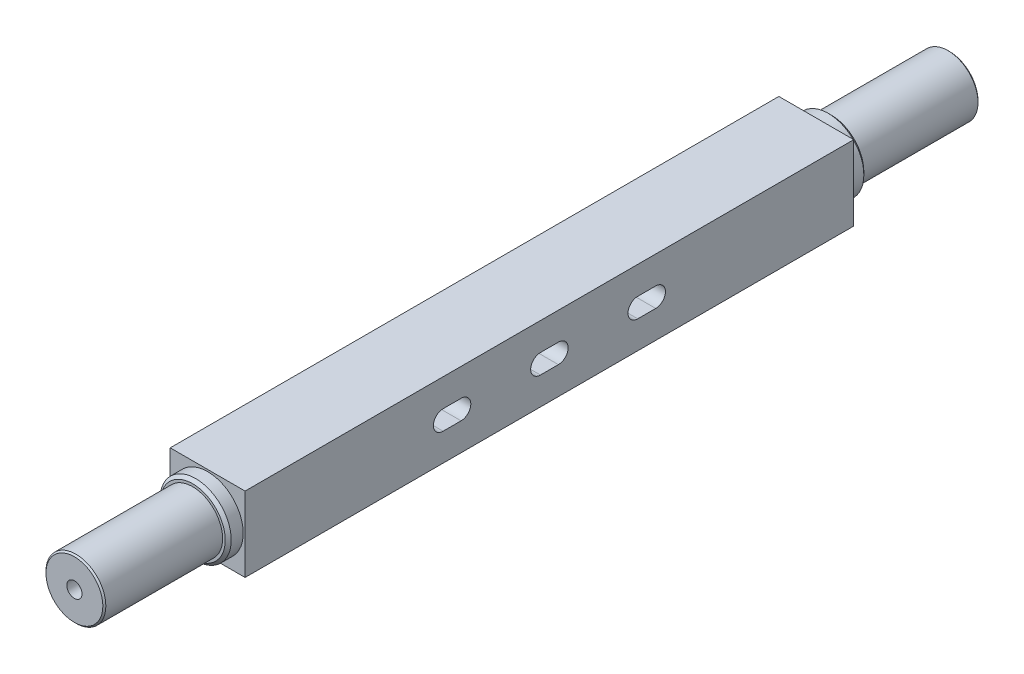
from build123d import *

# Parameters (mm, degrees)
SKETCH_1_R              = 20
EXTRUDE_1_DEPTH         = 79
SKETCH_2_R              = 23.75
EXTRUDE_2_DEPTH         = 10
CHAMFER_1_SIZE          = 2
SKETCH_3_W              = 50
SKETCH_3_H              = 50
EXTRUDE_3_DEPTH         = 406.5
SKETCH_4_R              = 23.75
EXTRUDE_4_DEPTH         = 10
CHAMFER_2_SIZE          = 2
SKETCH_5_R              = 20
EXTRUDE_5_DEPTH         = 79
CHAMFER_3_SIZE          = 1
HOLE_WIZARD_M12_1_D     = 10.2
HOLE_WIZARD_M12_1_DEPTH = 29.25
HOLE_WIZARD_M12_1_TIP   = 3.064389157
HOLE_WIZARD_M12_2_D     = 10.2
HOLE_WIZARD_M12_2_DEPTH = 29.25
HOLE_WIZARD_M12_2_TIP   = 3.064389157
CUT_EXTRUDE_1_DEPTH     = 79


with BuildPart() as part:
    # 草图1 → 凸台-拉伸1 (new body)
    with BuildSketch(Plane.XY):
        Circle(SKETCH_1_R)
    extrude(amount=EXTRUDE_1_DEPTH)

    # 草图2 → 凸台-拉伸2 (add)
    with BuildSketch(Plane.XY.offset(79)):
        Circle(SKETCH_2_R)
    extrude(amount=EXTRUDE_2_DEPTH)

    # 倒角1
    chamfer_1_edges = [part.edges().sort_by_distance(p)[0] for p in [
        (-23.75, 0, 79),
    ]]
    chamfer(chamfer_1_edges, length=CHAMFER_1_SIZE)

    # 草图3 → 凸台-拉伸3 (add)
    with BuildSketch(Plane.XY.offset(89)):
        Rectangle(SKETCH_3_W, SKETCH_3_H)
    extrude(amount=EXTRUDE_3_DEPTH)

    # 草图4 → 凸台-拉伸4 (add)
    with BuildSketch(Plane.XY.offset(495.5)):
        Circle(SKETCH_4_R)
    extrude(amount=EXTRUDE_4_DEPTH)

    # 倒角2
    chamfer_2_edges = [part.edges().sort_by_distance(p)[0] for p in [
        (-23.75, 0, 505.5),
    ]]
    chamfer(chamfer_2_edges, length=CHAMFER_2_SIZE)

    # 草图5 → 凸台-拉伸5 (add)
    with BuildSketch(Plane.XY.offset(505.5)):
        Circle(SKETCH_5_R)
    extrude(amount=EXTRUDE_5_DEPTH)

    # 倒角3
    chamfer_3_edges = [part.edges().sort_by_distance(p)[0] for p in [
        (-20, 0, 0),
        (-20, 0, 584.5),
    ]]
    chamfer(chamfer_3_edges, length=CHAMFER_3_SIZE)

    # M12 螺纹孔1
    with Locations(Plane(origin=(0, 0, 0), x_dir=(-1, 0, 0), z_dir=(0, 0, -1))):
        with Locations((0, 0)):
            Hole(HOLE_WIZARD_M12_1_D / 2, depth=HOLE_WIZARD_M12_1_DEPTH)
            with Locations((0, 0, -(HOLE_WIZARD_M12_1_DEPTH + HOLE_WIZARD_M12_1_TIP / 2))):  # 118° drill point
                Cone(0, HOLE_WIZARD_M12_1_D / 2, HOLE_WIZARD_M12_1_TIP, mode=Mode.SUBTRACT)

    # M12 螺纹孔2
    with Locations(Plane.XY.offset(584.5)):
        with Locations((0, 0)):
            Hole(HOLE_WIZARD_M12_2_D / 2, depth=HOLE_WIZARD_M12_2_DEPTH)
            with Locations((0, 0, -(HOLE_WIZARD_M12_2_DEPTH + HOLE_WIZARD_M12_2_TIP / 2))):  # 118° drill point
                Cone(0, HOLE_WIZARD_M12_2_D / 2, HOLE_WIZARD_M12_2_TIP, mode=Mode.SUBTRACT)

    # 草图10 → 切除-拉伸1 (cut)
    with BuildSketch(Plane(origin=(25, 0, 0), x_dir=(0, 0, -1), z_dir=(1, 0, 0))):
        with BuildLine():
            Line((-363.25, 6.5), (-351.25, 6.5))
            ThreePointArc((-351.25, 6.5), (-344.75, 0), (-351.25, -6.5))
            Line((-351.25, -6.5), (-363.25, -6.5))
            ThreePointArc((-363.25, -6.5), (-369.75, 0), (-363.25, 6.5))
        make_face()
        with BuildLine():
            Line((-298.25, 6.5), (-286.25, 6.5))
            ThreePointArc((-286.25, 6.5), (-279.75, 0), (-286.25, -6.5))
            Line((-286.25, -6.5), (-298.25, -6.5))
            ThreePointArc((-298.25, -6.5), (-304.75, 0), (-298.25, 6.5))
        make_face()
        with BuildLine():
            Line((-233.25, 6.5), (-221.25, 6.5))
            ThreePointArc((-221.25, 6.5), (-214.75, 0), (-221.25, -6.5))
            Line((-221.25, -6.5), (-233.25, -6.5))
            ThreePointArc((-233.25, -6.5), (-239.75, 0), (-233.25, 6.5))
        make_face()
    extrude(amount=-CUT_EXTRUDE_1_DEPTH, mode=Mode.SUBTRACT)


solid = part.part
